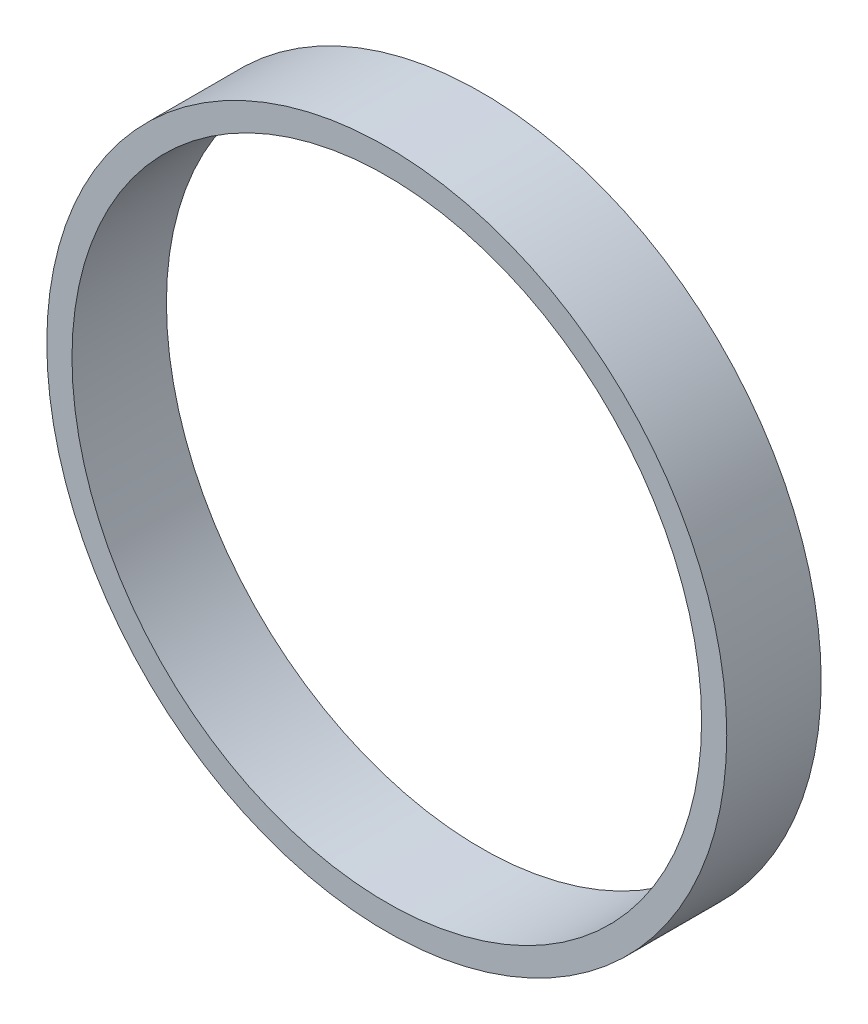
from build123d import *

# Parameters (mm, degrees)
SKETCH1_R           = 54
SKETCH1_R_2         = 50
BOSS_EXTRUDE1_DEPTH = 15


with BuildPart() as part:
    # Sketch1 → Boss-Extrude1 (new body)
    with BuildSketch(Plane.XY):
        Circle(SKETCH1_R)
        Circle(SKETCH1_R_2, mode=Mode.SUBTRACT)
    extrude(amount=BOSS_EXTRUDE1_DEPTH)


solid = part.part
